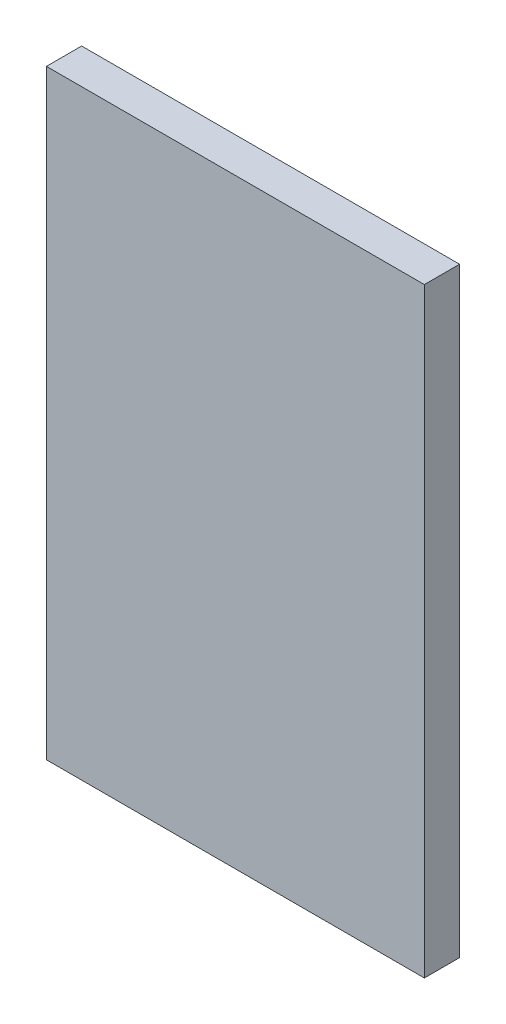
from build123d import *

# Parameters (mm, degrees)
SKETCH1_W           = 118
SKETCH1_H           = 187.5
BOSS_EXTRUDE1_DEPTH = 5.5


with BuildPart() as part:
    # Sketch1 → Boss-Extrude1 (new, symmetric)
    with BuildSketch(Plane.XY):
        Rectangle(SKETCH1_W, SKETCH1_H)
    extrude(amount=BOSS_EXTRUDE1_DEPTH, both=True)


solid = part.part
